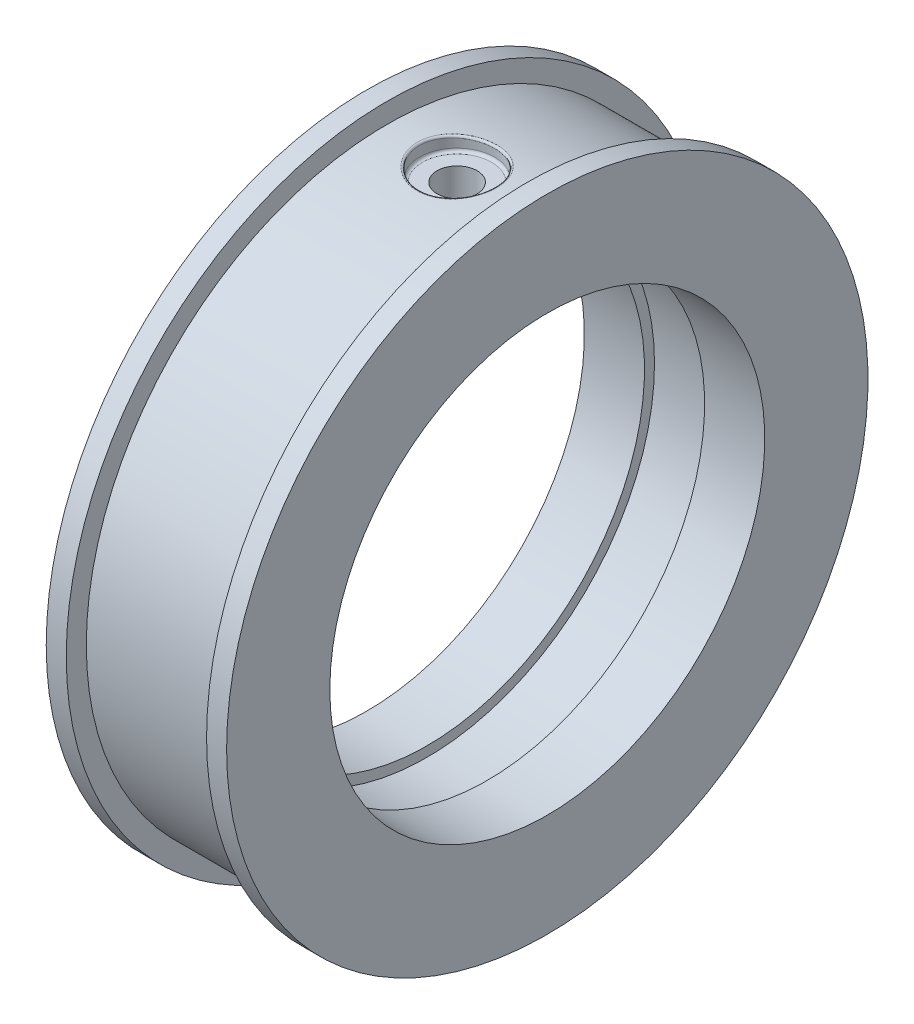
from build123d import *

# Parameters (mm, degrees)
HOLE1_D           = 7.5
HOLE1_DEPTH       = 1.5
HOLE2_REACH       = 71.113
HOLE2_BORE_R      = 2
DOWEL_HOLE1_D     = 4
DOWEL_HOLE1_DEPTH = 4
DOWEL_HOLE1_TIP   = 1.201721238
FILLET1_R         = 0.2
FILLET2_R         = 0.3


with BuildPart() as part:
    # Sketch1 → Revolve1 (revolve)
    with BuildSketch(Plane.XY, mode=Mode.PRIVATE) as revolve1_sk:
        Polygon((-8.389660143, 21.7), (-8.389660143, 32), (-6.389660143, 32), (-6.389660143, 30), (7.610339857, 30), (7.610339857, 32), (9.610339857, 32), (9.610339857, 21.7), (3.610339857, 21.7), (3.610339857, 22.7), (-2.389660143, 22.7), (-2.389660143, 21.7), align=None)
    revolve(revolve1_sk.sketch.rotate(Axis((-19.036826505, 0, 0), (1, 0, 0)), 90), axis=Axis((-19.036826505, 0, 0), (1, 0, 0)))

    # Hole1
    with Locations(Plane(origin=(0, 30, 0), x_dir=(1, 0, 0), z_dir=(0, 1, 0))):
        with Locations((0.610339857, 0)):
            Hole(HOLE1_D / 2, depth=HOLE1_DEPTH)

    # Hole2 bore → Hole2 (cut, up to next)
    with BuildSketch(Plane(origin=(0, 28.5, 0), x_dir=(1, 0, 0), z_dir=(0, 1, 0)), mode=Mode.PRIVATE) as hole2_sk1:
        with Locations((0.610339857, 0)):
            Circle(HOLE2_BORE_R)
    hole2_tool1 = extrude(hole2_sk1.sketch, amount=-HOLE2_REACH, mode=Mode.PRIVATE) & part.part
    add(hole2_tool1.solids().sort_by_distance((0.61034, 28.5, 0))[0], mode=Mode.SUBTRACT)

    # Dowel Hole1
    with Locations(Plane(origin=(0, -30, 0), x_dir=(-1, 0, 0), z_dir=(0, -1, 0))):
        with Locations((-0.610339857, 0)):
            Hole(DOWEL_HOLE1_D / 2, depth=DOWEL_HOLE1_DEPTH)
            with Locations((0, 0, -(DOWEL_HOLE1_DEPTH + DOWEL_HOLE1_TIP / 2))):  # 118° drill point
                Cone(0, DOWEL_HOLE1_D / 2, DOWEL_HOLE1_TIP, mode=Mode.SUBTRACT)

    # Fillet1
    fillet1_edges = [part.edges().sort_by_distance(p)[0] for p in [
        (4.360339864, 29.999999997, -1e-09),
    ]]
    fillet(fillet1_edges, radius=FILLET1_R)

    # Fillet2
    fillet2_edges = [part.edges().sort_by_distance(p)[0] for p in [
        (4.360339857, 28.5, 0),
    ]]
    fillet(fillet2_edges, radius=FILLET2_R)


solid = part.part
